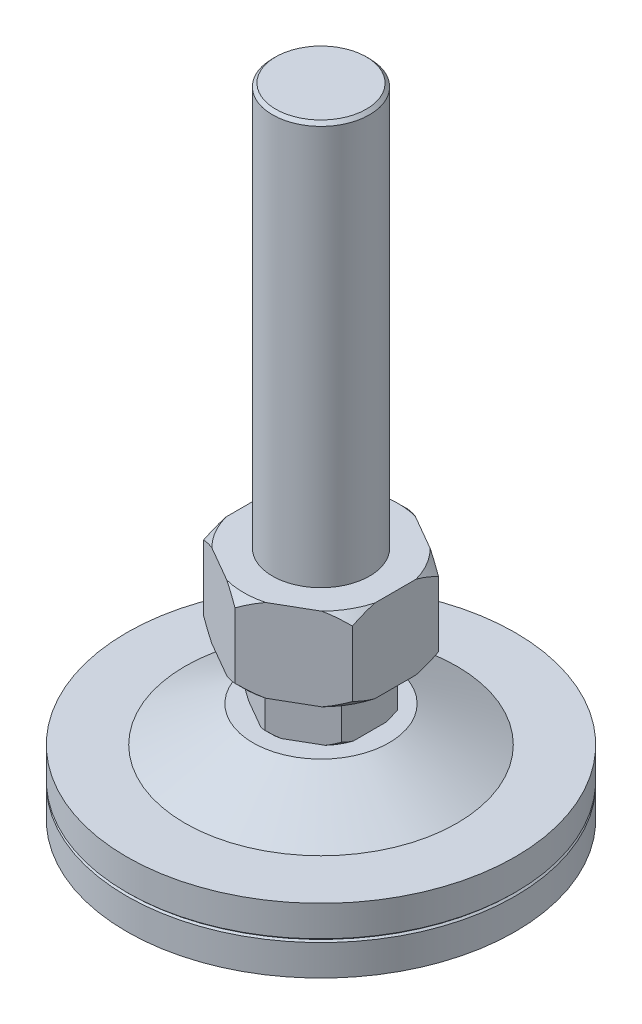
from build123d import *

# Parameters (mm, degrees)
BOSS_EXTRUDE1_DEPTH = 15
BOSS_EXTRUDE2_START = 25.6
SKETCH5_R           = 15
BOSS_EXTRUDE2_DEPTH = 25.6
CHAMFER1_SIZE       = 1


with BuildPart() as part:
    # Sketch1 → Revolve1 (revolve)
    with BuildSketch(Plane.XY, mode=Mode.PRIVATE) as revolve1_sk:
        Polygon((35, 0), (60, 0), (60, 9.5), (59.5, 10), (60, 10.5), (60, 20), (42, 20), (21, 31), (15, 31), (15, 197), (0, 197), (0, 15), (14, 15), align=None)
    revolve(revolve1_sk.sketch.rotate(Axis((0, 197, 0), (0, -1, 0)), 180), axis=Axis((0, 197, 0), (0, -1, 0)))

    # Sketch2 → Boss-Extrude1 (add)
    with BuildSketch(Plane(origin=(0, 31, 0), x_dir=(1, 0, 0), z_dir=(0, 1, 0))):
        Polygon((15, 8.660254038), (0, 17.320508076), (-15, 8.660254038), (-15, -8.660254038), (0, -17.320508076), (15, -8.660254038), align=None)
    extrude(amount=BOSS_EXTRUDE1_DEPTH)

    # Sketch3 → Cut-Revolve1 (revolve, cut)
    with BuildSketch(Plane(origin=(0, 0, 0), x_dir=(0, 0, -1), z_dir=(1, 0, 0))):
        Polygon((15.820508076, 31), (17.320508076, 32.5), (17.320508076, 31), align=None)
        Polygon((17.320508076, 44.5), (15.820508076, 46), (17.320508076, 46), align=None)
    revolve(axis=Axis((0, 197, 0), (0, 1, 0)), mode=Mode.SUBTRACT)

    # Sketch5 → Boss-Extrude2 (add)
    with BuildSketch(Plane(origin=(0, 47, 0), x_dir=(-1, 0, 0), z_dir=(0, 1, 0)).offset(BOSS_EXTRUDE2_START)):
        Polygon((0, 26.558112383), (-23, 13.279056191), (-23, -13.279056191), (0, -26.558112383), (23, -13.279056191), (23, 13.279056191), align=None)
        Circle(SKETCH5_R, mode=Mode.SUBTRACT)
    extrude(amount=-BOSS_EXTRUDE2_DEPTH)

    # Sketch7 → Cut-Revolve3 (revolve, cut)
    with BuildSketch(Plane(origin=(0, 0, 0), x_dir=(0, 0, -1), z_dir=(1, 0, 0))):
        Polygon((23.858112383, 72.6), (26.558112383, 69.9), (26.558112383, 72.6), align=None)
        Polygon((23.858112383, 47), (26.558112383, 49.7), (26.558112383, 47), align=None)
    revolve(axis=Axis((0, 197, 0), (0, 1, 0)), mode=Mode.SUBTRACT)

    # Chamfer1
    chamfer1_edges = [part.edges().sort_by_distance(p)[0] for p in [
        (15, 197, 0),
    ]]
    chamfer(chamfer1_edges, length=CHAMFER1_SIZE)


solid = part.part
